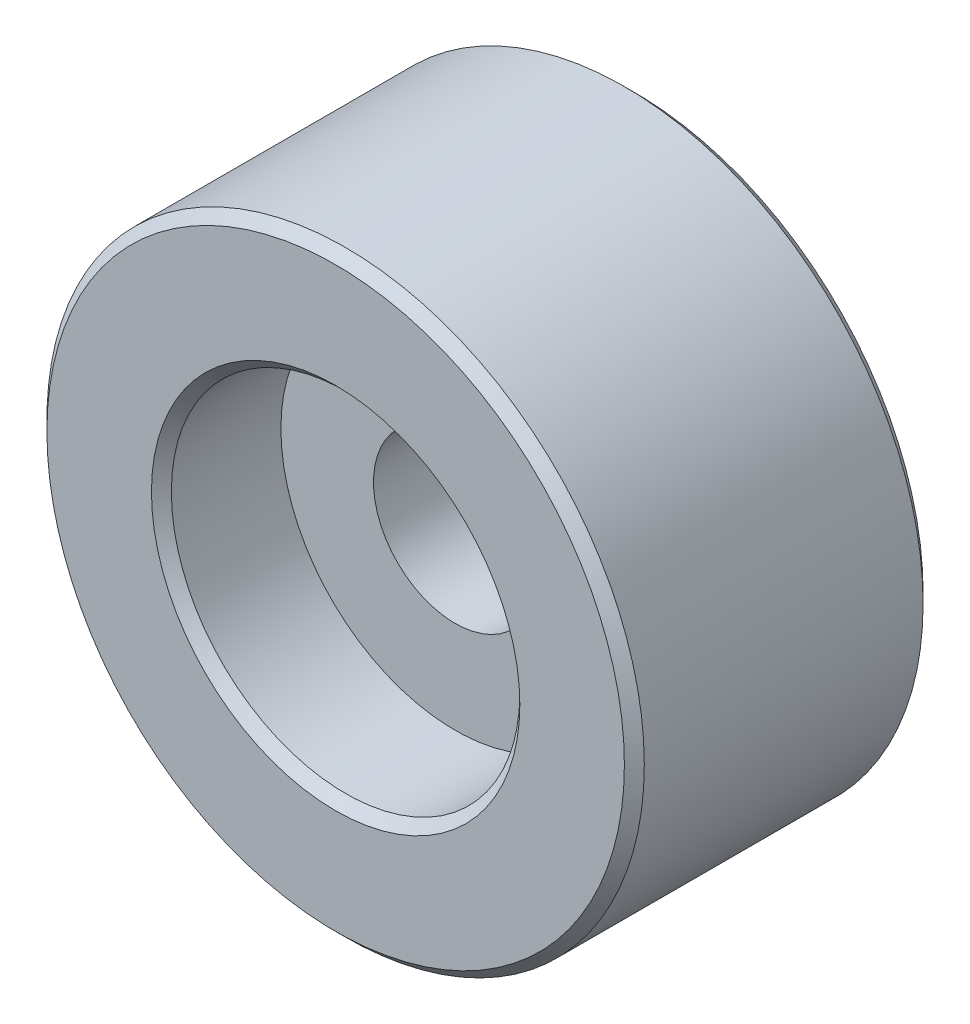
from build123d import *

# Parameters (mm, degrees)
SKETCH1_R           = 15
BOSS_EXTRUDE1_DEPTH = 15
SKETCH6_R           = 4.1
CUT_EXTRUDE3_DEPTH  = 50
SKETCH8_R           = 8.75
CUT_EXTRUDE5_DEPTH  = 6
CHAMFER2_SIZE       = 0.5
CHAMFER3_SIZE       = 0.5


with BuildPart() as part:
    # Sketch1 → Boss-Extrude1 (new body)
    with BuildSketch(Plane.XY):
        Circle(SKETCH1_R)
    extrude(amount=BOSS_EXTRUDE1_DEPTH)

    # Sketch6 → Cut-Extrude3 (cut)
    with BuildSketch(Plane(origin=(0, 0, 0), x_dir=(-1, 0, 0), z_dir=(0, 0, -1))):
        Circle(SKETCH6_R)
    extrude(amount=-CUT_EXTRUDE3_DEPTH, mode=Mode.SUBTRACT)

    # Sketch8 → Cut-Extrude5 (cut)
    with BuildSketch(Plane.XY.offset(15)):
        Circle(SKETCH8_R)
    extrude(amount=-CUT_EXTRUDE5_DEPTH, mode=Mode.SUBTRACT)

    # Chamfer2
    chamfer2_edges = [part.edges().sort_by_distance(p)[0] for p in [
        (-8.75, 0, 15),
    ]]
    chamfer(chamfer2_edges, length=CHAMFER2_SIZE)

    # Chamfer3
    chamfer3_edges = [part.edges().sort_by_distance(p)[0] for p in [
        (-15, 0, 0),
        (-15, 0, 15),
        (4.1, 0, 0),
    ]]
    chamfer(chamfer3_edges, length=CHAMFER3_SIZE)


solid = part.part
